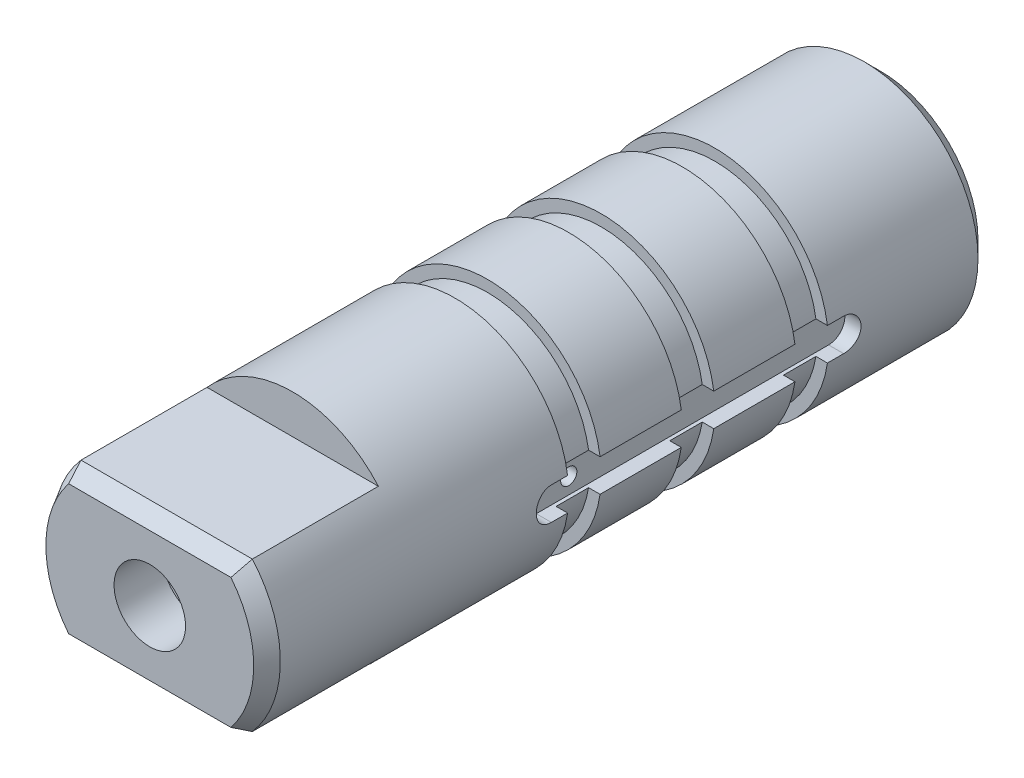
from build123d import *

# Parameters (mm, degrees)
SKETCH1_R                  = 35
BOSS_EXTRUDE1_DEPTH        = 112.5
SKETCH2_R                  = 35
SKETCH2_R_2                = 31.5
CUT_EXTRUDE1_DEPTH         = 5
LINEAR_PATTERN1_COUNT      = 2
LINEAR_PATTERN1_PITCH      = 35
LINEAR_PATTERN1_COL_COUNT  = 2
LINEAR_PATTERN1_COL_PITCH  = 35
CUT_EXTRUDE2_DEPTH         = 123.907485533
CUT_EXTRUDE2_DEPTH_BACK    = 123.907485533
BOSS_EXTRUDE2_DEPTH        = 30
CUT_EXTRUDE3_DEPTH         = 123.907485681
CUT_EXTRUDE3_DEPTH_BACK    = 123.907485681
SKETCH4_R                  = 2.5
CHAMFERC5_SIZE             = 5
CHAMFER3_30DEG_SIZE        = 3
CHAMFER3_30DEG_SIZE2       = 5.196152423
SKETCH5_W                  = 80
SKETCH5_H                  = 17
CUT_LEFT_PLANE_DEPTH       = 44
CHAMFER3_SIZE              = 3
CHAMFER3_SIZE2             = 5.196152423
M10X1_0_TAPPED_HOLE1_D     = 8
M10X1_0_TAPPED_HOLE1_DEPTH = 104
M10X1_0_TAPPED_HOLE1_TIP   = 2.403442476
SKETCH8_R                  = 11
CUT_EXTRUDE5_DEPTH         = 15


with BuildPart() as part:
    # Sketch1 → Boss-Extrude1 (new, symmetric)
    with BuildSketch(Plane.XY):
        Circle(SKETCH1_R)
    extrude(amount=BOSS_EXTRUDE1_DEPTH, both=True)

    # Sketch2 → Cut-Extrude1 (cut, symmetric)
    with BuildSketch(Plane.XY.offset(-21.5)):
        Circle(SKETCH2_R)
        Circle(SKETCH2_R_2, mode=Mode.SUBTRACT)
    cut_extrude1 = extrude(amount=CUT_EXTRUDE1_DEPTH, both=True, mode=Mode.SUBTRACT)

    # Linear pattern1: Cut-Extrude1 ×2
    with Locations(*[(0, 0, -i * LINEAR_PATTERN1_PITCH) for i in range(1, LINEAR_PATTERN1_COUNT)]):
        add(cut_extrude1, mode=Mode.SUBTRACT)

    # Linear pattern1 col: Cut-Extrude1 ×2
    with Locations(*[(0, 0, i * LINEAR_PATTERN1_COL_PITCH) for i in range(1, LINEAR_PATTERN1_COL_COUNT)]):
        add(cut_extrude1, mode=Mode.SUBTRACT)

    # Sketch3<2> → Cut-Extrude2 (cut, two sides: drawn at the far end of the back side and taken through both)
    with BuildSketch(Plane(origin=(0, 0, 0), x_dir=(0, 0, -1), z_dir=(1, 0, 0)).offset(-CUT_EXTRUDE2_DEPTH_BACK)):
        with BuildLine():
            Line((-23.5, 5), (66.5, 5))
            ThreePointArc((66.5, 5), (71.5, 0), (66.5, -5))
            Line((66.5, -5), (-23.5, -5))
            ThreePointArc((-23.5, -5), (-28.5, 0), (-23.5, 5))
        make_face()
    extrude(amount=CUT_EXTRUDE2_DEPTH + CUT_EXTRUDE2_DEPTH_BACK, mode=Mode.SUBTRACT)

    # 草图3<2> → Boss-Extrude2 (add, symmetric)
    with BuildSketch(Plane(origin=(0, 0, 0), x_dir=(0, 0, -1), z_dir=(1, 0, 0))):
        with BuildLine():
            Line((-23.5, 5), (66.5, 5))
            ThreePointArc((66.5, 5), (71.5, 0), (66.5, -5))
            Line((66.5, -5), (-23.5, -5))
            ThreePointArc((-23.5, -5), (-28.5, 0), (-23.5, 5))
        make_face()
    extrude(amount=BOSS_EXTRUDE2_DEPTH, both=True)

    # Sketch4 → Cut-Extrude3 (cut, two sides: drawn at the far end of the back side and taken through both)
    with BuildSketch(Plane(origin=(0, 0, 0), x_dir=(0, 0, -1), z_dir=(1, 0, 0)).offset(-CUT_EXTRUDE3_DEPTH_BACK)):
        with Locations((-13.5, 0)):
            Circle(SKETCH4_R)
    extrude(amount=CUT_EXTRUDE3_DEPTH + CUT_EXTRUDE3_DEPTH_BACK, mode=Mode.SUBTRACT)

    # ChamferC5
    chamferc5_edges = [part.edges().sort_by_distance(p)[0] for p in [
        (-35, 0, -112.5),
    ]]
    chamfer(chamferc5_edges, length=CHAMFERC5_SIZE)

    # Chamfer3-30deg
    chamfer3_30deg_edges = [part.edges().sort_by_distance(p)[0] for p in [
        (-35, 0, 112.5),
    ]]
    chamfer3_30deg_side = [part.faces().sort_by_distance(p)[0] for p in [
        (0, 0, 112.5),
    ]]
    chamfer(chamfer3_30deg_edges, length=CHAMFER3_30DEG_SIZE, length2=CHAMFER3_30DEG_SIZE2, reference=chamfer3_30deg_side[0])

    # Sketch5 → Cut-Left Plane (cut)
    with BuildSketch(Plane.XY.offset(112.5)):
        with Locations((0, 31.5)):
            Rectangle(SKETCH5_W, SKETCH5_H)
        with Locations((0, -31.5)):
            Rectangle(SKETCH5_W, SKETCH5_H)
    extrude(amount=-CUT_LEFT_PLANE_DEPTH, mode=Mode.SUBTRACT)

    # Chamfer3
    chamfer3_edges = [part.edges().sort_by_distance(p)[0] for p in [
        (0, -23, 112.5),
        (0, 23, 112.5),
    ]]
    chamfer3_side = [part.faces().sort_by_distance(p)[0] for p in [
        (0, 0, 112.5),
    ]]
    chamfer(chamfer3_edges, length=CHAMFER3_SIZE, length2=CHAMFER3_SIZE2, reference=chamfer3_side[0])

    # M10x1.0 Tapped Hole1
    with Locations(Plane.XY.offset(112.5)):
        with Locations((0, 0)):
            Hole(M10X1_0_TAPPED_HOLE1_D / 2, depth=M10X1_0_TAPPED_HOLE1_DEPTH)
            with Locations((0, 0, -(M10X1_0_TAPPED_HOLE1_DEPTH + M10X1_0_TAPPED_HOLE1_TIP / 2))):  # 118° drill point
                Cone(0, M10X1_0_TAPPED_HOLE1_D / 2, M10X1_0_TAPPED_HOLE1_TIP, mode=Mode.SUBTRACT)

    # Sketch8 → Cut-Extrude5 (cut)
    with BuildSketch(Plane.XY.offset(112.5)):
        Circle(SKETCH8_R)
    extrude(amount=-CUT_EXTRUDE5_DEPTH, mode=Mode.SUBTRACT)


solid = part.part
